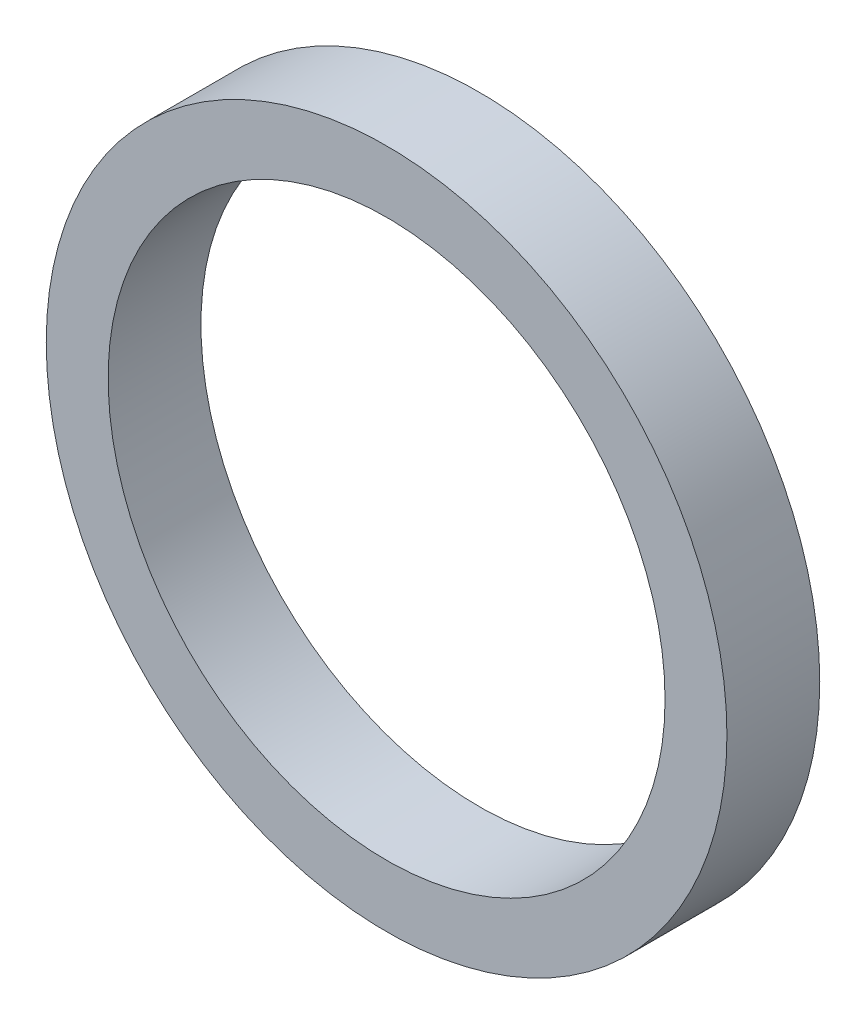
from build123d import *

# Parameters (mm, degrees)
SKETCH_1_R      = 110
SKETCH_1_R_2    = 90
EXTRUDE_2_DEPTH = 30


with BuildPart() as part:
    # 草图1 → 凸台-拉伸2 (new body)
    with BuildSketch(Plane.XY):
        Circle(SKETCH_1_R)
        Circle(SKETCH_1_R_2, mode=Mode.SUBTRACT)
    extrude(amount=EXTRUDE_2_DEPTH)


solid = part.part
